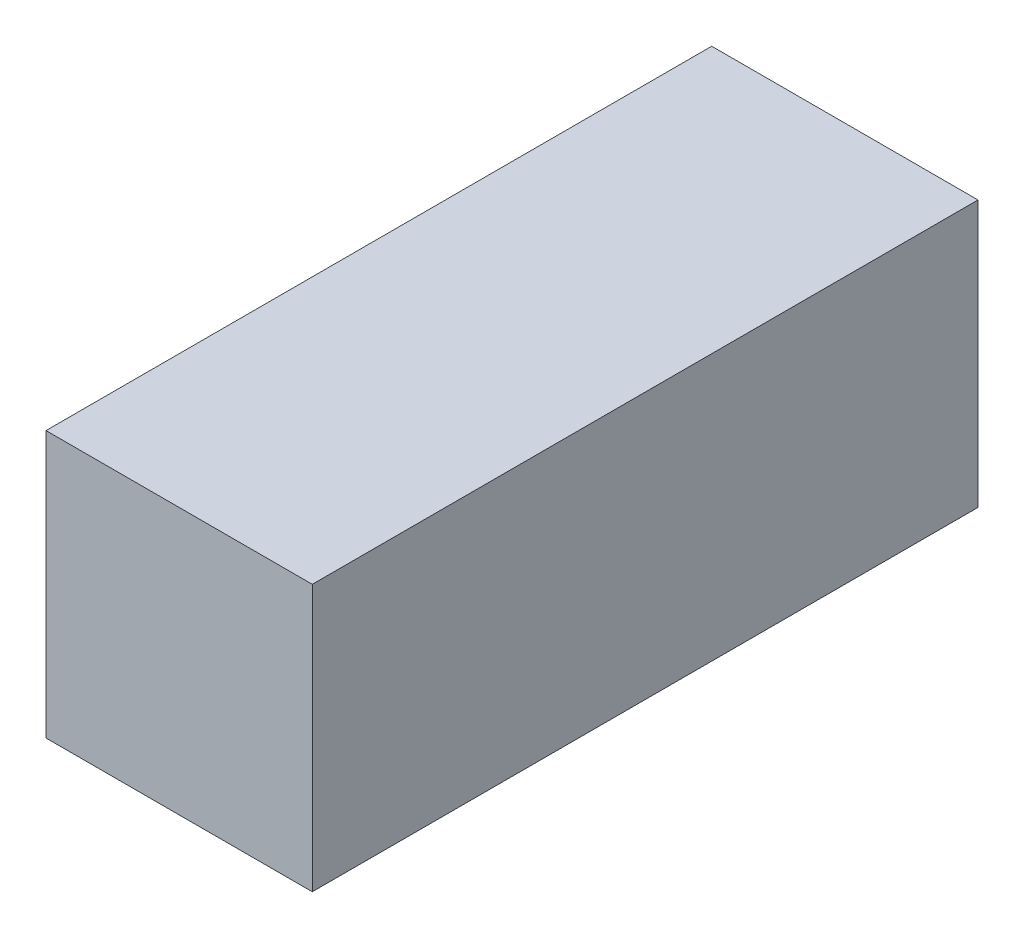
from build123d import *

# Parameters (mm, degrees)
SKETCH1_W           = 80
SKETCH1_H           = 80
BOSS_EXTRUDE1_DEPTH = 100


with BuildPart() as part:
    # Sketch1 → Boss-Extrude1 (new, symmetric)
    with BuildSketch(Plane.XY):
        Rectangle(SKETCH1_W, SKETCH1_H)
    extrude(amount=BOSS_EXTRUDE1_DEPTH, both=True)


solid = part.part
